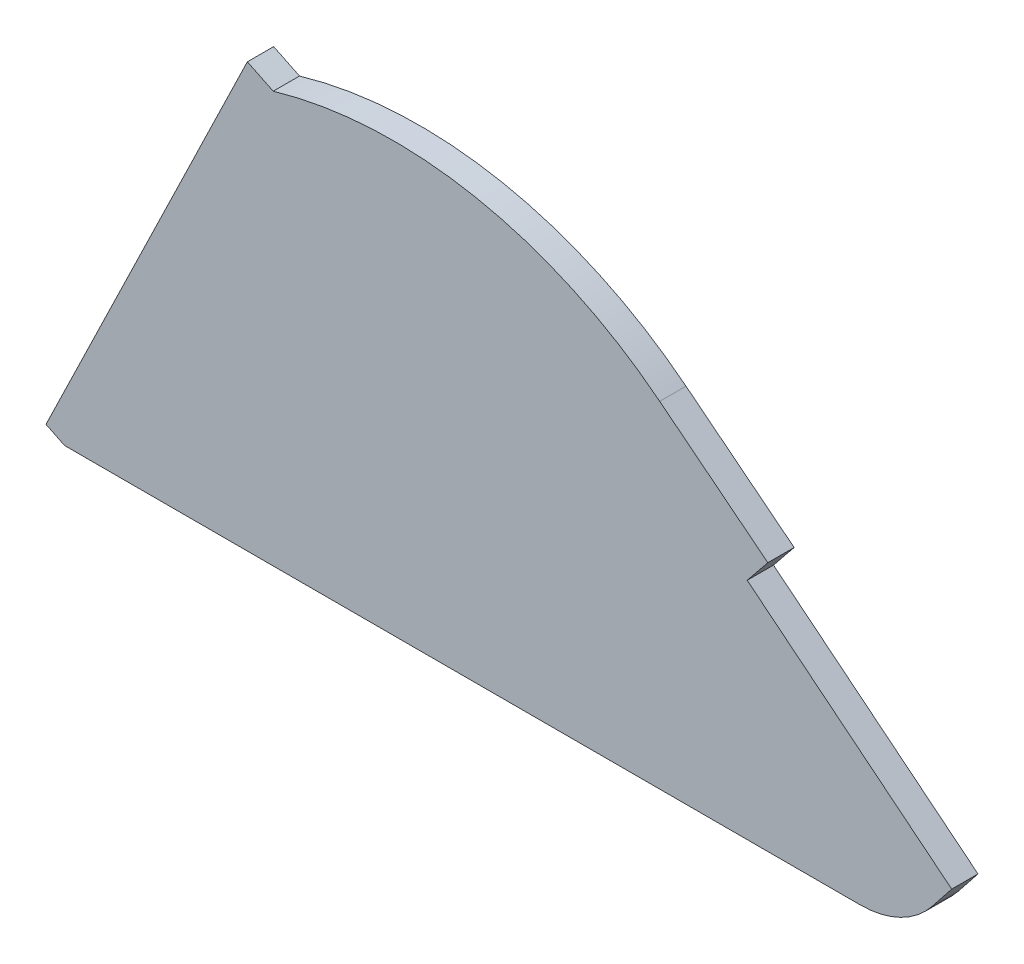
from build123d import *

# Parameters (mm, degrees)
BOSS_EXTRUDE1_DEPTH = 20


with BuildPart() as part:
    # Sketch1 → Boss-Extrude1 (new body)
    with BuildSketch(Plane.XY):
        with BuildLine():
            Line((0, 0), (605.341650479, 0))
            ThreePointArc((605.341650479, 0), (635.814099319, 6.980718334), (660.208845808, 26.53057538))
            Line((660.208845808, 26.53057538), (675, 45.2))
            Line((675, 45.2), (519.4, 170.9))
            Line((519.4, 170.9), (535.110173103, 190.347119609))
            Line((535.110173103, 190.347119609), (452.843320373, 255.524366816))
            ThreePointArc((452.843320373, 255.524366816), (312.777423466, 319.976650776), (158.75851208, 312.854339417))
            Line((158.75851208, 312.854339417), (139.1, 322.4))
            Line((139.1, 322.4), (-14.119827283, 6.856219748))
            Line((-14.119827283, 6.856219748), (0, 0))
        make_face()
    extrude(amount=BOSS_EXTRUDE1_DEPTH)


solid = part.part
